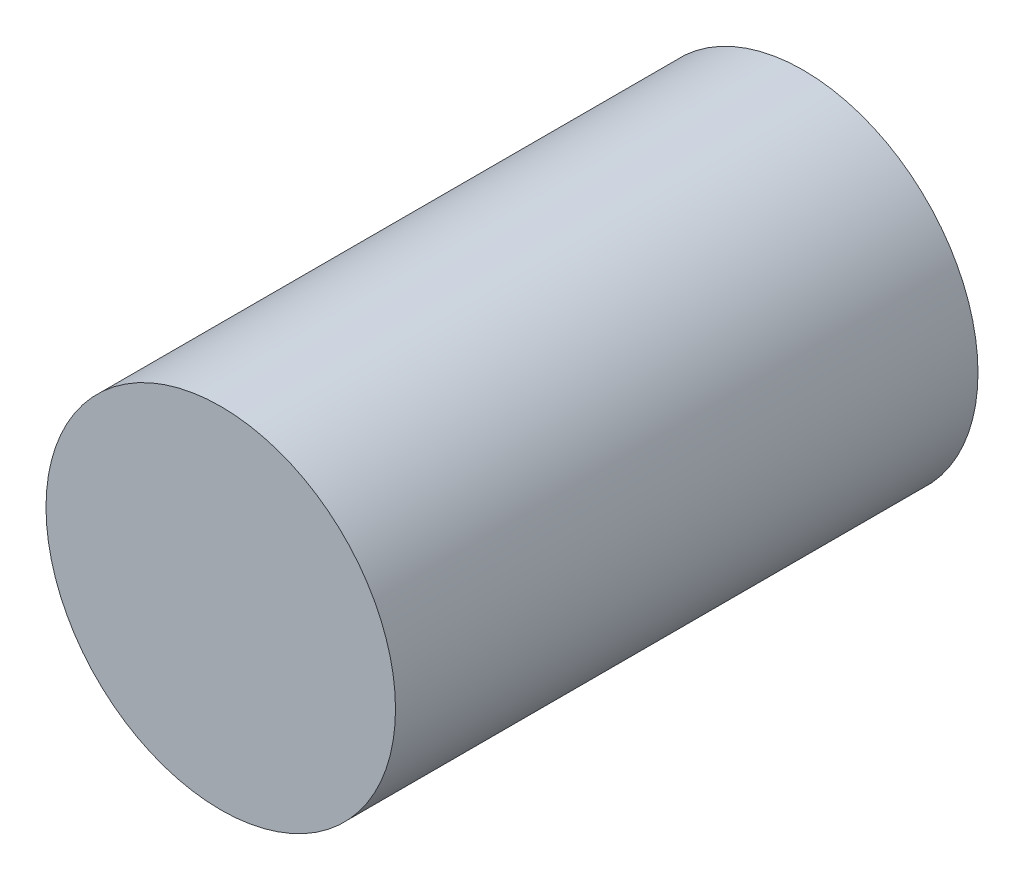
SolidWorks part; units mm, degrees
material "6061 合金"
ref_plane "前视基准面" through (0, 0, 0) normal (0, 0, 1) x (1, 0, 0)
ref_plane "上视基准面" through (0, 0, 0) normal (0, 1, 0) x (1, 0, 0)
ref_plane "右视基准面" through (0, 0, 0) normal (1, 0, 0) x (0, 0, -1)
sketch "草图1" plane through (0, 0, 0) normal (0, 0, 1) x (1, 0, 0)
  circle A0 centre (0, 0) radius 7.5
  dimension "D1" = 15
extrude "凸台-拉伸1" add sketch "草图1" along normal blind 25
sketch "草图4" plane through (0, 0, 0) normal (0, 0, -1) x (-1, 0, 0)
  point P0 (0, 0)
hole_wizard "M4 螺纹孔1" positions "草图4" profile "草图3" tap size "M4" standard "GB"
sketch "草图3" plane through (0, 0, 0) normal (1, 0, 0) x (0, 1, 0)
  line L0 (0, 0) -> (0, 11.0914)
  line L1 (0, 11.0914) -> (1.65, 10.1)
  line L2 (1.65, 10.1) -> (1.65, 0)
  line L5 (1.65, 0) -> (0, 0)
  line L10 (0, 11.0914) -> (-1.65, 10.1) construction
  line L11 (0, -6.35) -> (0, 107.95) construction
  dimension "螺纹孔钻头直径" = 3.3
  dimension "螺纹孔钻头深度" = 10.1
  dimension "导头角度" = 118
cosmetic thread "孔螺纹线1" parameters "D1"=8, "D2"=4
